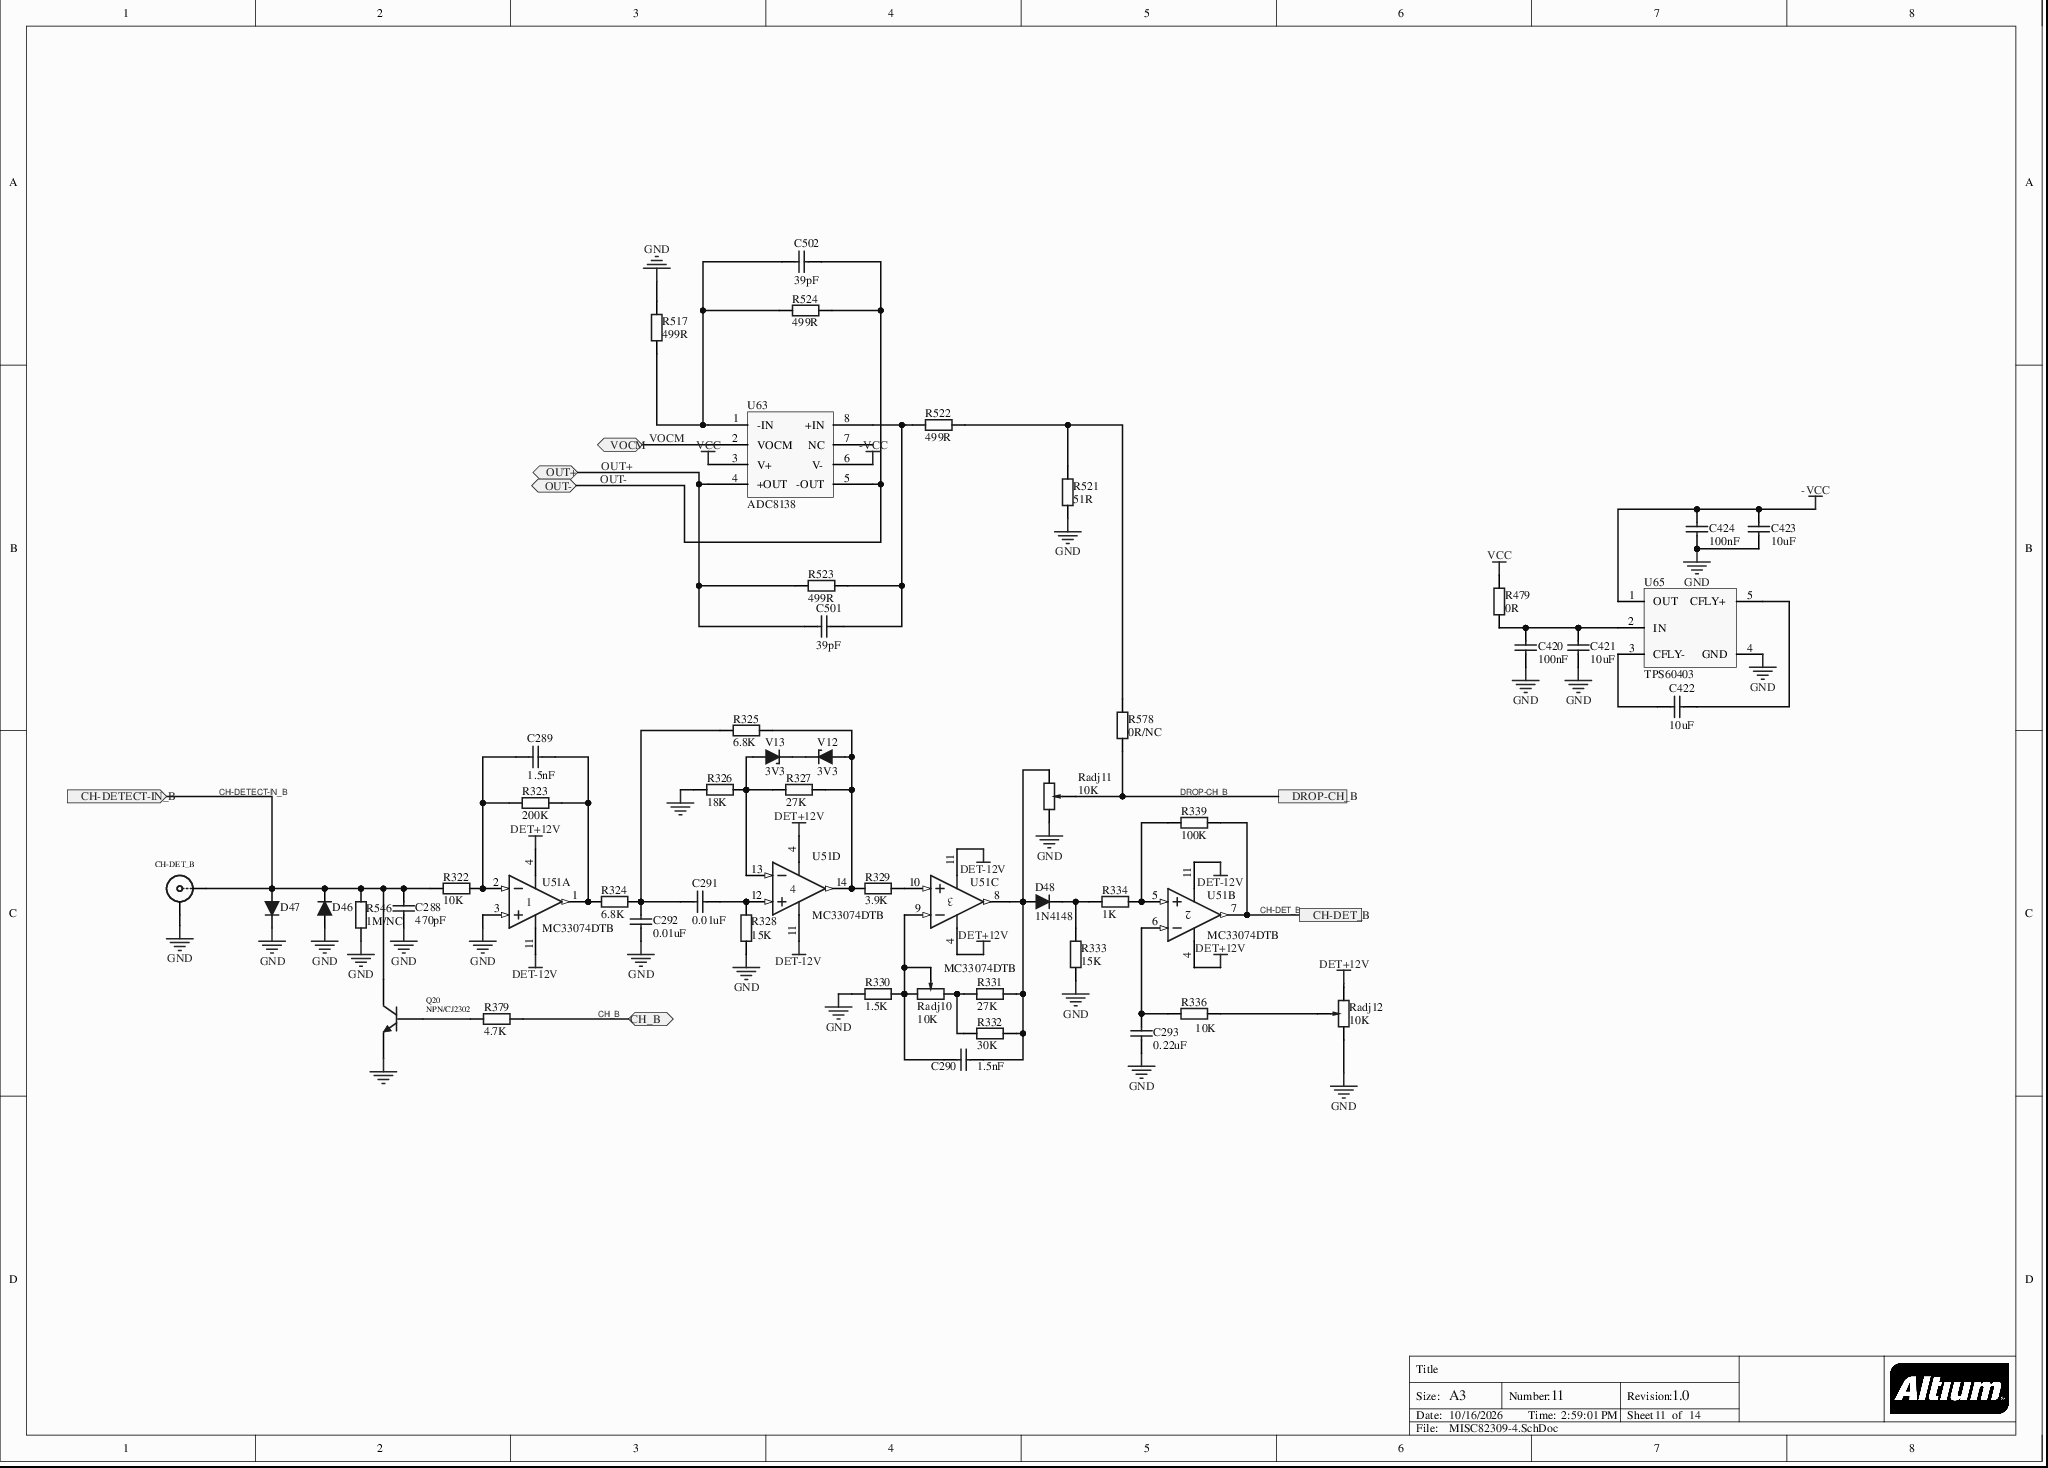
[diagram p0: MISC82309-4.SchDoc]
# Altium project MISC82309-16.PrjPcb (part 5 of 6)

## Sheet MISC82309-4.SchDoc
size A3; DocumentNumber: 11; Revision: 1.0; SheetNumber: 11; SheetTotal: 14

### Parts
C288  470pF  [C0603]
C289  1.5nF  [C0603]
C290  1.5nF  [C0603]
C291  0.01uF  [C0603]
C292  0.01uF  [C0603]
C293  0.22uF  [C0603]
C420  100nF  [CAP_0603]
C421  10uF  [CAP_0603]
C422  10uF  [CAP_0603]
C423  10uF  [CAP_0603]
C424  100nF  [CAP_0603]
C501  39pF  [CAP_0603]
C502  39pF  [CAP_0603]
CH-DET_B  SMB  [SMB_V-RJ45]  (value not drawn)
D46  1N4148WS  [SOD323]  (value not drawn)
D47  1N4148WS  [SOD323]  (value not drawn)
D48  1N4148  [SOD-323]
Q20  NPN/CJ2302  [SOT-23-3]
R322  10K  [RES_0603]
R323  200K  [RES_0603]
R324  6.8K  [RES_0603]
R325  6.8K  [RES_0603]
R326  18K  [RES_0603]
R327  27K  [RES_0603]
R328  15K  [RES_0603]
R329  3.9K  [RES_0603]
R330  1.5K  [RES_0603]
R331  27K  [RES_0603]
R332  30K  [RES_0603]
R333  15K  [RES_0603]
R334  1K  [RES_0603]
R336  10K  [RES_0603]
R339  100K  [RES_0603]
R379  4.7K  [RES_0603]
R479  0R  [RES_0603]
R517  499R  [RES_0603]
R521  51R  [RES_0603]
R522  499R  [RES_0603]
R523  499R  [RES_0603]
R524  499R  [RES_0603]
R546  1M/NC  [RES_0603]
R578  0R/NC  [RES_0603]
Radj10  10K  [Radj]
Radj11  10K  [Radj]
Radj12  10K  [Radj]
U51  MC33074DTB  [948G-01_N]  (parts A,B,C,D of 4)
U63  ADC8138  [SO8_N]
U65  TPS60403  [SOT23-5_M]
V12  3V3  [SOD-123]
V13  3V3  [SOD-123]

### Ports
CH-DET_B, CH-DETECT-IN_B (in), CH_B (bidir), DROP-CH_B, OUT+ (bidir), OUT- (bidir), VOCM (bidir)

### Nets
-VCC: C423.1 C424.2 U63.6(V-) U65.1(OUT)
DET+12V: Radj12.3 U51.4(V+)
DET-12V: U51.11(V-)
GND: C288.1 C292.2 C293.2 C420.1 C421.1 C423.2 C424.1 CH-DET_B.2(Y) D46.1 D47.2 Q20.2(E) R326.1 R328.1 R330.1 R333.1 R517.2 R521.2 R546.1 Radj11.1 Radj12.1 U51.3(IN+) U65.4(GND)
VCC: R479.2 U63.3(V+)
CH-DET_B: R339.2 U51.7(OUT) ; port CH-DET_B
CH-DETECT-IN_B: C288.2 CH-DET_B.1(X) D46.2 D47.1 Q20.3(C) R322.1 R546.2 ; port CH-DETECT-IN_B
CH_B: R379.2 ; port CH_B
DROP-CH_B: R578.1 Radj11.2 ; port DROP-CH_B
OUT+: C501.1 R523.1 U63.4(+OUT) ; port OUT+
OUT-: C502.1 R524.1 U63.5(-OUT) ; port OUT-
VOCM: U63.2(VOCM) ; port VOCM
NetC289_1: C289.1 R323.2 R324.1 U51.1(OUT)
NetC289_2: C289.2 R322.2 R323.1 U51.2(IN-)
NetC290_1: C290.1 D48.1 R331.2 R332.2 Radj11.3 U51.8(OUT)
NetC290_2: C290.2 R330.2 Radj10.2 Radj10.3 U51.9(IN-)
NetC291_1: C291.1 R328.2 U51.12(IN+)
NetC291_2: C291.2 C292.1 R324.2 R325.1
NetC293_1: C293.1 R336.1 U51.6(IN-)
NetC420_2: C420.2 C421.2 R479.1 U65.2(IN)
NetC422_1: C422.1 U65.5(CFLY+)
NetC422_2: C422.2 U65.3(CFLY-)
NetC501_2: C501.2 R522.1 R523.2 U63.8(+IN)
NetC502_2: C502.2 R517.1 R524.2 U63.1(-IN)
NetD48_2: D48.2 R333.2 R334.1
NetQ20_1: Q20.1(B) R379.1
NetR325_2: R325.2 R327.2 R329.2 U51.14(OUT) V12.1
NetR326_2: R326.2 R327.1 U51.13(IN-) V13.1
NetR329_1: R329.1 U51.10(IN+)
NetR331_1: R331.1 R332.1 Radj10.1
NetR334_2: R334.2 R339.1 U51.5(IN+)
NetR336_2: R336.2 Radj12.2
NetR521_1: R521.1 R522.2 R578.2
NetV12_2: V12.2 V13.2

Not connected (* = marked no-connect by the designer): U63 7(NC)

### Notes on the sheet
- Title
- Size:
- Date:
- A3
- Number:
- Time:
- Revision:
- Sheet
- of
- File:

### Library data of the parts
C288-C293 C421-C423 C501 C502 = CAP_0603: Capacitor
  C288: value: 470pF
  C289 C290: value: 1.5nF
  C291 C292: value: 0.01uF
  C293: value: 0.22uF
  C421-C423: value: 10uF
  C501 C502: value: 39pF
C420 C424 = CAP_0603: Capacitor; value: 39pF
CH-DET_B = SMB: SMB Straight Connector; LatestRevisionDate: 17-Jul-2002; LatestRevisionNote: Re-released for DXP Platform.; PCB DECAL: SMB_V-RJ45; Comment_1: SMB; Publisher: Altium Limited
D48 = Diode-SMD
Q20 = NPN: Value: NPN/CJ2302
R322-R329 R331-R334 R336 R339 R379 R479 R517 R521-R524 R546 R578 = Res_0603: Res
  R322 R336: value: 10K
  R323: value: 200K
  R324 R325: value: 6.8K
  R326: value: 18K
  R327 R331: value: 27K
  R328 R333: value: 15K
  R329: value: 3.9K
  R332: value: 30K
  R334: value: 1K
  R339: value: 100K
  R379: value: 4.7K
  R479: value: 0R
  R517 R522-R524: value: 499R
  R521: value: 51R
  R546: value: 1M/NC
  R578: value: 0R/NC
R330 = Res_0603: Res; value: 10K
Radj10-Radj12 = Radj: value: 10K
U51 = MC33074DTB: Single-Supply 3 to 44 V Operational Amplifier; Published: 28-Feb-2003; LatestRevisionDate: 12-Dec-2006; LatestRevisionNote: IPC-7351 Footprint Added.; DatasheetVersion: Jan-2002, Rev. 5; PackageVersion: 1998; PackageReference: 948G-01; PackageDescription: 14-Pin Thin Small Outline Package 0.65 mm Pitch; ComponentLink1Description: Manufacturer Link; ComponentLink1URL: http://www.onsemi.com/; ComponentLink2Description: Datasheet; ComponentLink2URL: http://www.onsemi.com/pub/Collateral/MC34071-D.PDF; Publisher: Altium Limited
U63 = AD8138
V12 V13 = BZT52C3V3

## Sheet MISC82309-14.SchDoc
size A4; Revision: 1.0; SheetNumber: 12; SheetTotal: 14
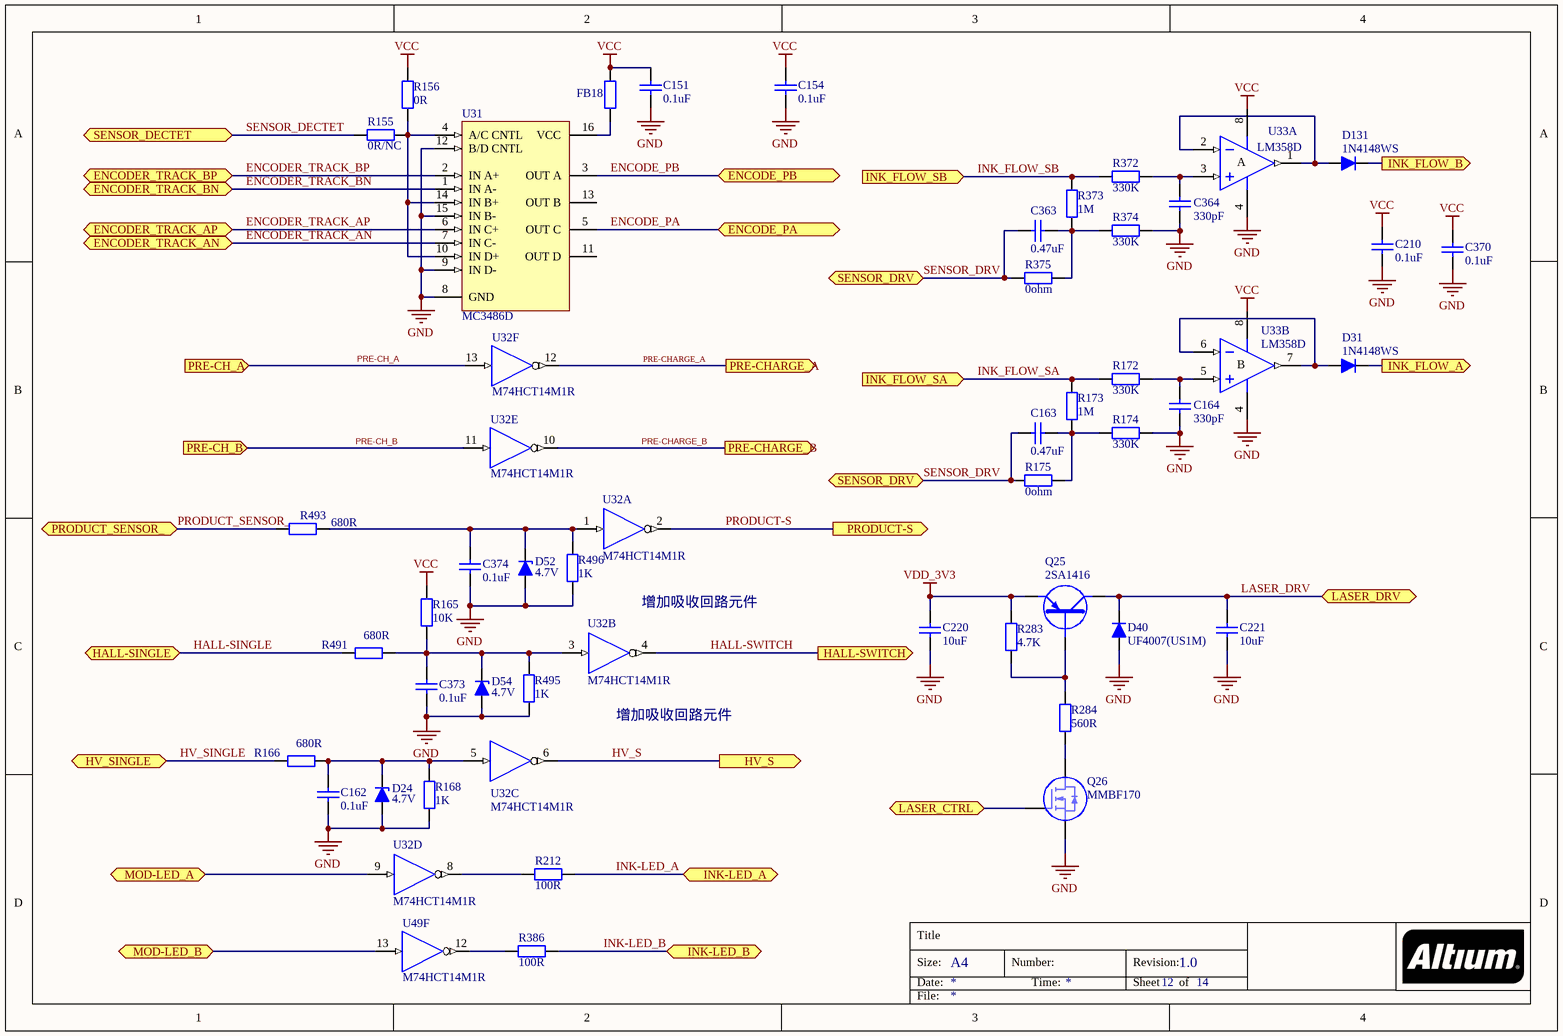
[diagram p1: MISC82309-14.SchDoc]

### Parts
C151  0.1uF  [CAP_0805]
C154  0.1uF  [CAP_0805]
C162  0.1uF  [CAP_0805]
C163  0.47uF  [C0603]
C164  330pF  [C0603]
C210  0.1uF  [CAP_0603]
C220  10uF  [CAP_0805]
C221  10uF  [CAP_0805]
C363  0.47uF  [C0603]
C364  330pF  [C0603]
C370  0.1uF  [CAP_0603]
C373  0.1uF  [CAP_0805]
C374  0.1uF  [CAP_0805]
D24  4.7V  [SOD-123]
D31  1N4148WS  [SOD323]
D40  UF4007(US1M)  [DO-214AA]
D52  4.7V  [SOD-123]
D54  4.7V  [SOD-123]
D131  1N4148WS  [SOD323]
FB18  60  [SMD0805-L]  (value not drawn)
Q25  2SA1416  [SOT89]
Q26  MMBF170  [SOT-23]
R155  0R/NC  [R0805]
R156  0R  [R0805]
R165  10K  [R0805]
R166  680R  [R0805]
R168  1K  [R0805]
R172  330K  [R0603]
R173  1M  [R0603]
R174  330K  [R0603]
R175  0ohm  [R0603]
R212  100R  [R0805]
R283  4.7K  [R0805]
R284  560R  [R0805]
R372  330K  [R0603]
R373  1M  [R0603]
R374  330K  [R0603]
R375  0ohm  [R0603]
R386  100R  [R0805]
R491  680R  [R0805]
R493  680R  [R0805]
R495  1K  [R0805]
R496  1K  [R0805]
U31  MC3486D  [751B-03]
U32  M74HCT14M1R  [SO14_N]  (parts A,B,C,D,E,F of 6)
U33  LM358D  [SO8_N]  (parts A,B of 2)
U49  M74HCT14M1R  [SO14_N]  (part F of 6)

### Ports
ENCODE_PA, ENCODE_PB, ENCODER_TRACK_AN, ENCODER_TRACK_AP, ENCODER_TRACK_BN, ENCODER_TRACK_BP, HALL-SINGLE (bidir), HALL-SWITCH (out), HV_S (out), HV_SINGLE (bidir), INK-LED_A, INK-LED_B, INK_FLOW_A (out), INK_FLOW_B (out), INK_FLOW_SA (in), INK_FLOW_SB (in), LASER_CTRL, LASER_DRV, MOD-LED_A, MOD-LED_B, PRE-CH_A, PRE-CH_B, PRE-CHARGE_A (out), PRE-CHARGE_B (out), PRODUCT-S (out), PRODUCT_SENSOR_, SENSOR_DECTET, SENSOR_DRV (bidir)

### Nets
GND: C151.1 C154.1 C162.1 C164.1 C210.1 C220.1 C221.1 C364.1 C370.1 C373.1 C374.1 D24.1 D40.1 D52.1 D54.1 Q26.2(S) R168.1 R174.2 R374.2 R495.1 R496.1 U31.8(GND) U31.9(IN_D-) U31.12(B/D_CNTL) U31.15(IN_B-) U32.7(GND) U33.4(V-) U49.7(GND)
VCC: C151.2 C154.2 C210.2 C370.2 FB18.2 R156.2 R165.2 U32.14(VCC) U33.8(V+) U49.14(VCC)
VDD_3V3: C220.2 Q25.3(E) R283.2
ENCODE_PA: U31.5(OUT_C) ; port ENCODE_PA
ENCODE_PB: U31.3(OUT_A) ; port ENCODE_PB
ENCODER_TRACK_AN: U31.7(IN_C-) ; port ENCODER_TRACK_AN
ENCODER_TRACK_AP: U31.6(IN_C+) ; port ENCODER_TRACK_AP
ENCODER_TRACK_BN: U31.1(IN_A-) ; port ENCODER_TRACK_BN
ENCODER_TRACK_BP: U31.2(IN_A+) ; port ENCODER_TRACK_BP
HALL-SINGLE: R491.1 ; port HALL-SINGLE
HALL-SWITCH: U32.4(Y) ; port HALL-SWITCH
HV_S: U32.6(Y) ; port HV_S
HV_SINGLE: R166.1 ; port HV_SINGLE
INK-LED_A: R212.2 ; port INK-LED_A
INK-LED_B: R386.2 ; port INK-LED_B
INK_FLOW_A: D31.2 ; port INK_FLOW_A
INK_FLOW_B: D131.2 ; port INK_FLOW_B
INK_FLOW_SA: R172.2 R173.2 ; port INK_FLOW_SA
INK_FLOW_SB: R372.2 R373.2 ; port INK_FLOW_SB
LASER_CTRL: Q26.1(G) ; port LASER_CTRL
LASER_DRV: C221.2 D40.2 Q25.2(C) ; port LASER_DRV
MOD-LED_A: U32.9(A) ; port MOD-LED_A
MOD-LED_B: U49.13(A) ; port MOD-LED_B
PRE-CH_A: U32.13(A) ; port PRE-CH_A
PRE-CH_B: U32.11(A) ; port PRE-CH_B
PRE-CHARGE_A: U32.12(Y) ; port PRE-CHARGE_A
PRE-CHARGE_B: U32.10(Y) ; port PRE-CHARGE_B
PRODUCT-S: U32.2(Y) ; port PRODUCT-S
PRODUCT_SENSOR_: R493.1 ; port PRODUCT_SENSOR_
SENSOR_DECTET: R155.1 ; port SENSOR_DECTET
SENSOR_DRV: C163.2 C363.2 R175.1 R375.1 ; port SENSOR_DRV
NetC162_2: C162.2 D24.2 R166.2 R168.2 U32.5(A)
NetC163_1: C163.1 R173.1 R174.1 R175.2
NetC164_2: C164.2 R172.1 U33.5(IN+)
NetC363_1: C363.1 R373.1 R374.1 R375.2
NetC364_2: C364.2 R372.1 U33.3(IN+)
NetC373_2: C373.2 D54.2 R165.1 R491.2 R495.2 U32.3(A)
NetC374_2: C374.2 D52.2 R493.2 R496.2 U32.1(A)
NetD31_1: D31.1 U33.6(IN-) U33.7(OUT)
NetD131_1: D131.1 U33.1(OUT) U33.2(IN-)
NetFB18_1: FB18.1 U31.16(VCC)
NetQ25_1: Q25.1 R283.1 R284.2
NetQ26_3: Q26.3(D) R284.1
NetR155_2: R155.2 R156.1 U31.4(A/C_CNTL) U31.10(IN_D+) U31.14(IN_B+)
NetR212_1: R212.1 U32.8(Y)
NetR386_1: R386.1 U49.12(Y)

Not connected (* = marked no-connect by the designer): U31 11(OUT_D) 13(OUT_B)

### Notes on the sheet
- (near U32) 增加吸收回路元件
- 增加吸收回路元件
- Title
- Size:
- Date:
- A4
- Number:
- Time:
- Revision:
- Sheet
- of
- File:

### Library data of the parts
C151 C154 C162 C220 C221 C373 C374 = CAP_0805: Capacitor
  C151 C154 C162 C373 C374: value: 0.1uF
  C220 C221: value: 10uF
C163 C164 C363 C364 = Cap: Capacitor; Published: 8-Jun-2000; LatestRevisionDate: 17-Jul-2002; LatestRevisionNote: Re-released for DXP Platform.; PackageReference: RAD-0.3; Publisher: Altium Limited
  C163 C363: Value: 0.47uF
  C164 C364: Value: 330pF
C210 C370 = CAP_0603: Capacitor; value: 0.1uF
D24 D52 D54 = BZT52C4V7
D40 = UF4007
FB18 = FB: Res; value: 10K
Q26 = MOSFET-N: N-Channel MOSFET; Published: 8-Jun-2000; LatestRevisionDate: 17-Jul-2002; LatestRevisionNote: Re-released for DXP Platform.; PackageVersion: 1995/1996; PackageReference: E3; PackageDescription: TO, Flat Index; 3 In-Line, Axial Leads; Body Dia. 4.6mm; Lead Dia. 0.5 mm (max); Publisher: Altium Limited
R155 R156 R165 R166 R168 R212 R283 R284 R386 R491 R493 R495 R496 = Res_0805: Res
  R155: value: 0R/NC
  R156: value: 0R
  R165: value: 10K
  R166 R491 R493: value: 680R
  R168 R495 R496: value: 1K
  R212 R386: value: 100R
  R283: value: 4.7K
  R284: value: 560R
R172-R175 R372-R375 = Res2: Resistor; Published: 8-Jun-2000; LatestRevisionDate: 17-Jul-2002; LatestRevisionNote: Re-released for DXP Platform.; PackageReference: AXIAL-0.4; Publisher: Altium Limited
  R172 R174 R372 R374: Value: 330K
  R173 R373: Value: 1M
  R175 R375: Value: 0ohm
U31 = MC3486D: Quad EIA-422/423 Line Receiver; Published: 17-Jul-2002; LatestRevisionDate: 13-Apr-2006; LatestRevisionNote: IPC-7351 Footprint Added.; DatasheetVersion: 1988; PackageVersion: 1991; PackageReference: 751B-03; PackageDescription: 16-Pin Small Outline Integrated Circuit 1.27 mm Pitch; Code_JEDEC: MS-012-AC; Code_IPC: SOIC127P600-16; ComponentLink1Description: Manufacturer Link; ComponentLink1URL: http://www.onsemi.com/site/products/parametrics/0,4446,178,00.html; Publisher: Altium Limited
U32 U49 = M74HCT14M1R: Hex Schmitt Inverter; Published: 8-Jun-2000; LatestRevisionDate: 13-Apr-2006; LatestRevisionNote: IPC-7351 Footprint Added.; DatasheetVersion: Oct-1993; PackageVersion: Sep-1998; PackageReference: SO14; PackageDescription: 14-Pin Small Outline Integrated Circuit 1.27 mm Pitch; Code_IPC: SOIC127P600-14; ComponentLink1Description: Manufacturer Link; ComponentLink1URL: http://www.st.com/; ComponentLink2Description: Datasheet; ComponentLink2URL: http://www.st.com/stonline/products/literature/ds/2106/m74hct14.pdf; Publisher: Altium Limited
U33 = LM358D: Dual Low-Power Operational Amplifier; Published: 24-Aug-2001; LatestRevisionDate: 13-Apr-2006; LatestRevisionNote: IPC-7351 Footprint Added.; PackageVersion: Dec-2002; PackageReference: SO8; PackageDescription: 8-Pin Small Outline Integrated Circuit 1.27 mm Pitch; Code_JEDEC: MS-012-AA; Code_IPC: SOIC127P600-8; ComponentLink1Description: Manufacturer Link; ComponentLink1URL: http://www.st.com/; ComponentLink2Description: Datasheet; ComponentLink2URL: http://www.st.com/stonline/products/literature/ds/2163/lm358.pdf; Publisher: Altium Limited

## Sheet MISC82309-9.SchDoc
size A4; DocumentNumber: 13; Revision: 1.0; SheetNumber: 13; SheetTotal: 14
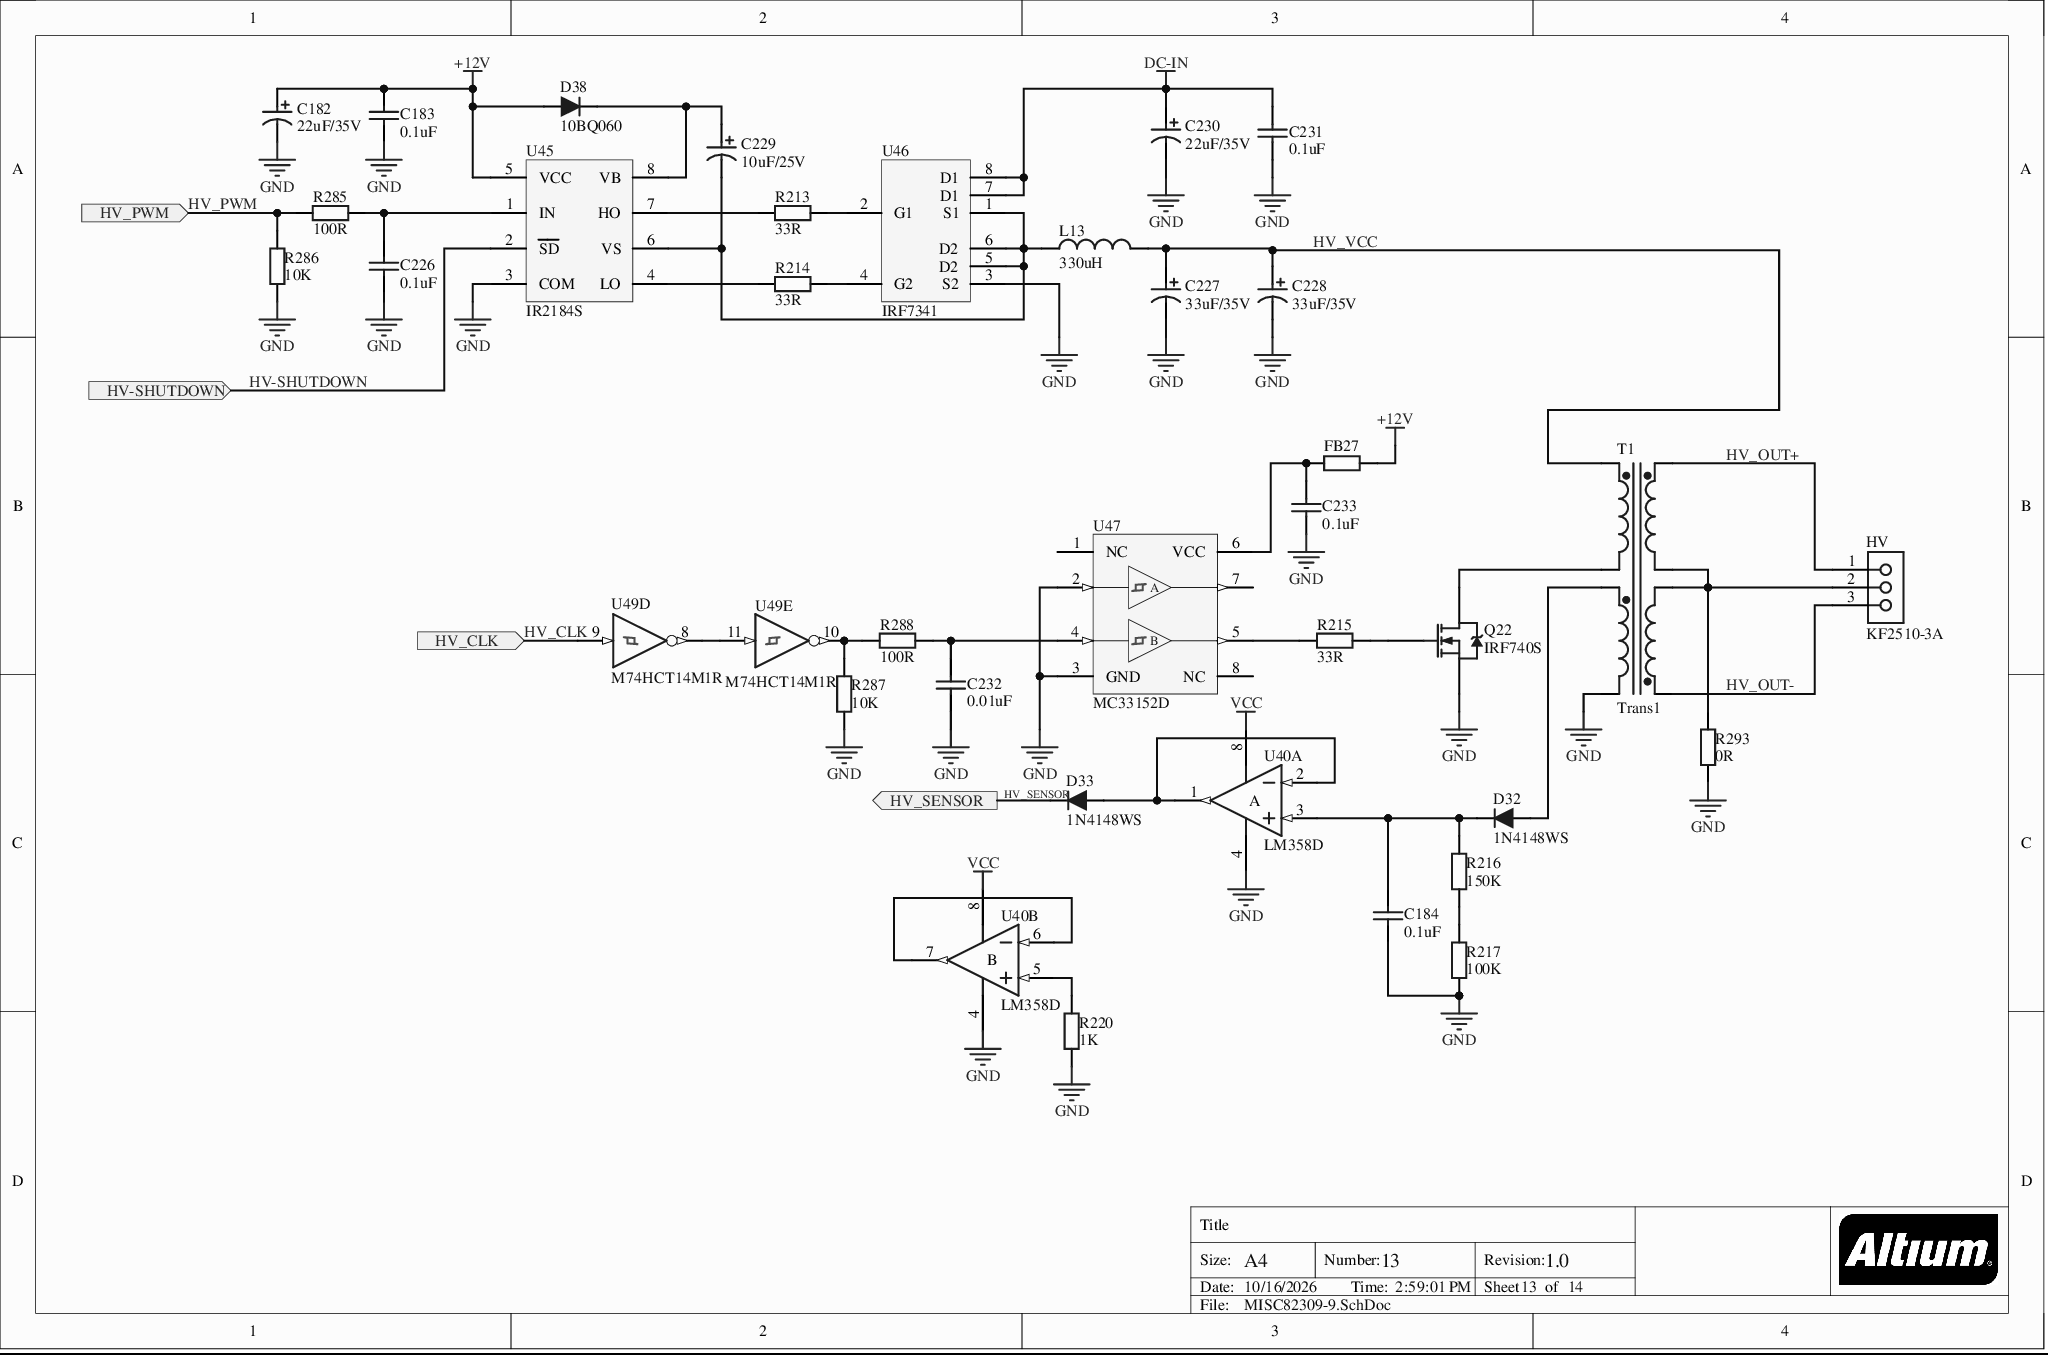
[diagram p2: MISC82309-9.SchDoc]

### Parts
C182  22uF/35V  [CAP-ALU-6_3X5_4]
C183  0.1uF  [CAP_0805]
C184  0.1uF  [CAP_0805]
C226  0.1uF  [CAP_0603]
C227  33uF/35V  [CAP-ALU-6_3X5_4]
C228  33uF/35V  [CAP-ALU-6_3X5_4]
C229  10uF/25V  [CAP-ALU-5X5_4]
C230  22uF/35V  [CAP-ALU-6_3X5_4]
C231  0.1uF  [CAP_0805]
C232  0.01uF  [CAP_0603]
C233  0.1uF  [CAP_0805]
D32  1N4148WS  [SOD323]
D33  1N4148WS  [SOD323]
D38  10BQ060  [DO-214AA-L]
FB27  60  [SMD0805-L]  (value not drawn)
HV  KF2510-3A  [KF2510-3A]
L13  330uH  [PBS5022]
Q22  IRF740S  [D2PAK_N]
R213  33R  [RES_0603]
R214  33R  [RES_0603]
R215  33R  [RES_0805]
R216  150K  [R0805]
R217  100K  [R0805]
R220  1K  [R0805]
R285  100R  [RES_0603]
R286  10K  [RES_0603]
R287  10K  [RES_0603]
R288  100R  [RES_0603]
R293  0R  [RES_0805]
T1  Trans1  [RM8]
U40  LM358D  [SO8_N]  (parts A,B of 2)
U45  IR2184S  [SOIC_8N]
U46  IRF7341  [SOIC_8N]
U47  MC33152D  [751-05_N]
U49  M74HCT14M1R  [SO14_N]  (parts D,E of 6)

### Ports
HV-SHUTDOWN (in), HV_CLK (in), HV_PWM (in), HV_SENSOR (out)

### Nets
+12V: C182.2 C183.2 D38.1 FB27.2 U45.5(VCC)
DC-IN: C230.2 C231.2 U46.7(D1) U46.8(D1)
GND: C182.1 C183.1 C184.1 C226.1 C227.1 C228.1 C230.1 C231.1 C232.1 C233.1 Q22.3(S) R217.2 R220.2 R286.1 R287.1 R293.2 T1.3(F+) U40.4(V-) U45.3(COM) U46.3(S2) U47.2(INA) U47.3(GND) U49.7(GND)
VCC: U40.8(V+) U49.14(VCC)
HV-SHUTDOWN: U45.2(~{SD}) ; port HV-SHUTDOWN
HV_CLK: U49.9(A) ; port HV_CLK
HV_OUT+: HV.1 T1.7(Sec1+)
HV_OUT-: HV.3 T1.8(Sec2-)
HV_PWM: R285.1 R286.2 ; port HV_PWM
HV_SENSOR: D33.2 ; port HV_SENSOR
HV_VCC: C227.2 C228.2 L13.2 T1.2(Pri-)
NetC184_2: C184.2 D32.2 R216.2 U40.3(IN+)
NetC226_2: C226.2 R285.2 U45.1(IN)
NetC229_1: C229.1 L13.1 U45.6(VS) U46.1(S1) U46.5(D2) U46.6(D2)
NetC229_2: C229.2 D38.2 U45.8(VB)
NetC232_2: C232.2 R288.2 U47.4(INB)
NetC233_2: C233.2 FB27.1 U47.6(VCC)
NetD32_1: D32.1 T1.4(F-)
NetD33_1: D33.1 U40.1(OUT) U40.2(IN-)
NetHV_2: HV.2 R293.1 T1.11(Sec1-) T1.12(Sec2+)
NetQ22_1: Q22.1(G) R215.1
NetQ22_2: Q22.2(D) T1.1(Pri+)
NetR213_1: R213.1 U46.2(G1)
NetR213_2: R213.2 U45.7(HO)
NetR214_1: R214.1 U46.4(G2)
NetR214_2: R214.2 U45.4(LO)
NetR215_2: R215.2 U47.5(~{OUTB})
NetR216_1: R216.1 R217.1
NetR220_1: R220.1 U40.5(IN+)
NetR287_2: R287.2 R288.1 U49.10(Y)
NetU40_6: U40.6(IN-) U40.7(OUT)
NetU49_8: U49.8(Y) U49.11(A)

Not connected (* = marked no-connect by the designer): U47 1(NC) 7(~{OUTA}) 8(NC)

### Notes on the sheet
- Title
- Size:
- Date:
- A4
- Number:
- Time:
- Revision:
- Sheet
- of
- File:

### Library data of the parts
C182 C227-C230 = CAP_ALU: Capacitor
  C182 C230: value: 22uF/35V
  C227 C228: value: 33uF/35V
  C229: value: 10uF/25V
C183 C184 C231 C233 = CAP_0805: Capacitor; value: 0.1uF
C226 C232 = CAP_0603: Capacitor
  C226: value: 0.1uF
  C232: value: 0.01uF
FB27 = FB: Res; value: 10K
L13 = Inductor: value: 330uH
Q22 = IRF740S: HEXFET N-Channel Power MOSFET; Published: 8-Jun-2000; LatestRevisionDate: 20-Nov-2009; LatestRevisionNote: IPC-7351 Footprint Added.; DatasheetVersion: PD-9.1010; PackageReference: D2PAK; PackageDescription: 3-Pin Transistor Outline Package 2.54 mm Pitch, 15.1 mm Lead Span; ComponentLink1Description: Manufacturer Link; ComponentLink1URL: http://www.irf.com/; ComponentLink2Description: Datasheet; ComponentLink2URL: http://www.irf.com/product-info/datasheets/data/irf740s.pdf; Publisher: Altium Limited
R213 R214 R285-R288 = Res_0603: Res
  R213 R214: value: 33R
  R285 R288: value: 100R
  R286 R287: value: 10K
R215 R217 R220 R293 = Res_0805: Res
  R215: value: 33R
  R217: value: 100K
  R220: value: 1K
  R293: value: 0R
R216 = Res_0805: Res; value: 4.7K
T1 = Trans1: Three-winding Transformer (Non-Ideal); Sim Note: Enter the turns ratios, Core loss resistance, Magnetising Reactance, Leakage Reactances and Resistances referred to the primary side into the parameter fields.; Published: 25-Jan-2001; LatestRevisionDate: 17-Jul-2002; LatestRevisionNote: Re-released for DXP Platform.; PackageReference: TRF_6; PackageDescription: Transformer; 6 Leads; Publisher: Altium Limited
U40 = LM358D: Dual Low-Power Operational Amplifier; Published: 24-Aug-2001; LatestRevisionDate: 13-Apr-2006; LatestRevisionNote: IPC-7351 Footprint Added.; PackageVersion: Dec-2002; PackageReference: SO8; PackageDescription: 8-Pin Small Outline Integrated Circuit 1.27 mm Pitch; Code_JEDEC: MS-012-AA; Code_IPC: SOIC127P600-8; ComponentLink1Description: Manufacturer Link; ComponentLink1URL: http://www.st.com/; ComponentLink2Description: Datasheet; ComponentLink2URL: http://www.st.com/stonline/products/literature/ds/2163/lm358.pdf; Publisher: Altium Limited
U47 = MC33152D: High Speed Dual MOSFET Driver; Published: 17-Jul-2002; LatestRevisionDate: 13-Apr-2006; LatestRevisionNote: IPC-7351 Footprint Added.; DatasheetVersion: 1996; PackageVersion: 1996; PackageReference: 751-05; PackageDescription: 8-Pin Small Outline Integrated Circuit 1.27 mm Pitch; Code_JEDEC: MS-012-AA; Code_IPC: SOIC127P600-8; ComponentLink1Description: Manufacturer Link; ComponentLink1URL: http://www.onsemi.com/site/products/parametrics/0,4446,388,00.html; ComponentLink2Description: Datasheet; ComponentLink2URL: http://www.onsemi.com/pub/Collateral/MC34152-D.PDF; Publisher: Altium Limited
U49 = M74HCT14M1R: Hex Schmitt Inverter; Published: 8-Jun-2000; LatestRevisionDate: 13-Apr-2006; LatestRevisionNote: IPC-7351 Footprint Added.; DatasheetVersion: Oct-1993; PackageVersion: Sep-1998; PackageReference: SO14; PackageDescription: 14-Pin Small Outline Integrated Circuit 1.27 mm Pitch; Code_IPC: SOIC127P600-14; ComponentLink1Description: Manufacturer Link; ComponentLink1URL: http://www.st.com/; ComponentLink2Description: Datasheet; ComponentLink2URL: http://www.st.com/stonline/products/literature/ds/2106/m74hct14.pdf; Publisher: Altium Limited